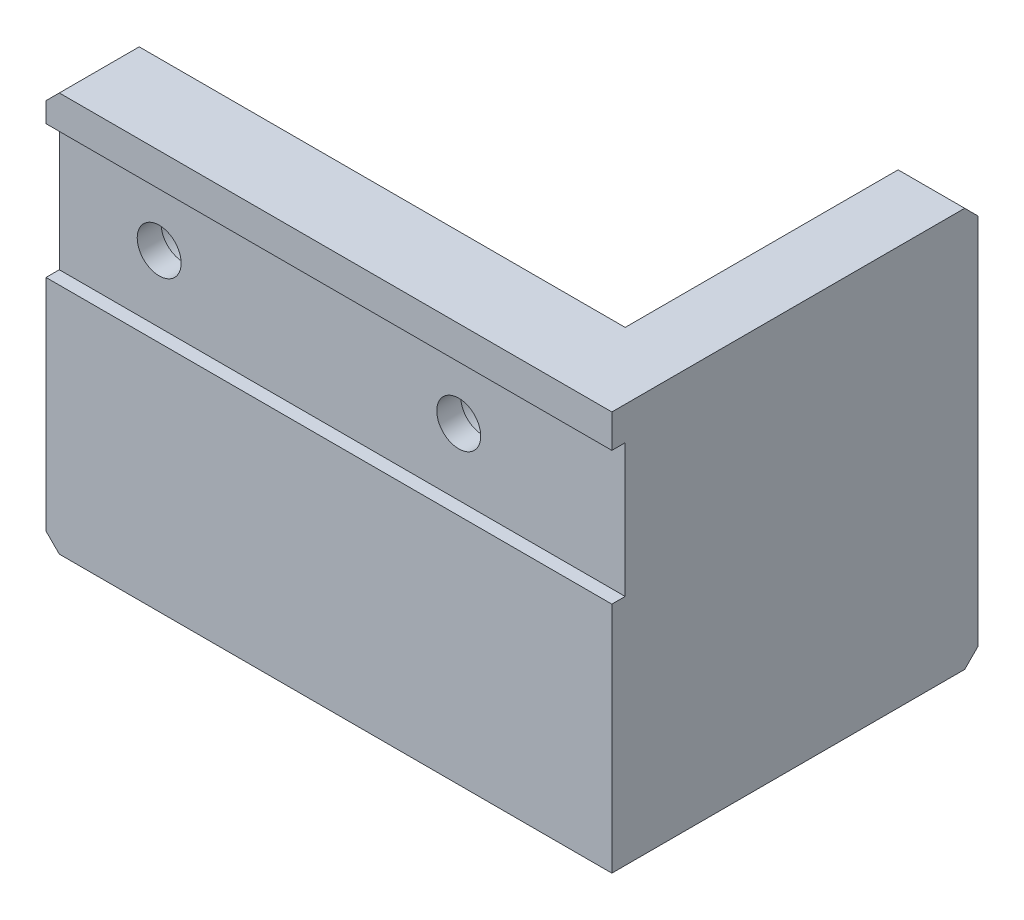
SolidWorks part; units mm, degrees
material "6061-T6"
ref_plane "前视基准面" through (0, 0, 0) normal (0, 0, 1) x (1, 0, 0)
ref_plane "上视基准面" through (0, 0, 0) normal (0, 1, 0) x (1, 0, 0)
ref_plane "右视基准面" through (0, 0, 0) normal (1, 0, 0) x (0, 0, -1)
sketch "草图2" plane through (0, 0, 0) normal (0, 0, 1) x (1, 0, 0)
  line L1 (0, 0) -> (90, 0)
  line L2 (0, 0) -> (0, -60)
  line L3 (0, -60) -> (90, -60)
  line L4 (90, 0) -> (90, -60)
  dimension "D1" = 90
  dimension "D2" = 60
extrude "凸台-拉伸1" add sketch "草图2" along normal blind 12
sketch "草图3" plane through (90, 0, 0) normal (1, 0, 0) x (0, 0, -1)
  line L6 (-12, -60) -> (-12, 0) construction
  line L7 (-12, -5) -> (-10, -5)
  line L8 (-12, -5) -> (-12, -25)
  line L9 (-12, -25) -> (-10, -25)
  line L10 (-10, -5) -> (-10, -25)
  line L12 (-12, 0) -> (0, 0) construction
  dimension "D1" = 2
  dimension "D2" = 5
  dimension "D3" = 20
extrude "切除-拉伸1" cut sketch "草图3" against normal through all
sketch "草图4" plane through (0, 0, 0) normal (0, 1, 0) x (1, 0, 0)
  line L0 (90, 0) -> (0, 0) construction
  line L1 (75, 0) -> (85, 0)
  line L2 (75, 0) -> (75, -1)
  line L3 (75, -1) -> (85, -1)
  line L4 (85, 0) -> (85, -1)
  line L5 (90, -12) -> (90, 0) construction
  dimension "D1" = 1
  dimension "D2" = 5
  dimension "D3" = 10
extrude "切除-拉伸2" cut sketch "草图4" against normal through all
hole_wizard "M6 六角凹头螺钉的柱形沉头孔4" positions "草图5" profile "草图6" counterbore size "M6" standard "ISO"
sketch "草图5" plane through (0, 0, 10) normal (0, 0, 1) x (1, 0, 0)
  line L1 (90, -25) -> (90, -5) construction
  line L2 (80, -15) -> (90, -15) construction
  point P0 (80, -15)
  dimension "D1" = 10
sketch "草图6" plane through (80, -15, 10) normal (1, 0, 0) x (0, -1, 0)
  line L0 (0, 0) -> (0, 18.9828)
  line L1 (0, 18.9828) -> (3.3, 17)
  line L2 (3.3, 17) -> (3.3, 6.4)
  line L3 (3.3, 6.4) -> (5.5, 6.4)
  line L4 (5.5, 6.4) -> (5.5, 0)
  line L5 (5.5, 0) -> (0, 0)
  line L10 (0, 18.9828) -> (-3.3, 17) construction
  line L11 (0, -6.35) -> (0, 107.95) construction
  dimension "孔直径" = 6.6
  dimension "孔深度" = 17
  dimension "柱形沉头孔直径" = 11
  dimension "柱形沉头孔深度" = 6.4
  dimension "导头角度" = 118
hole_wizard "M6 六角凹头螺钉的柱形沉头孔5" positions "草图7" profile "草图8" counterbore size "M6" standard "ISO"
sketch "草图7" plane through (0, 0, 12) normal (0, 0, 1) x (1, 0, 0)
  line L0 (80, -15) -> (80, -45) construction
  line L2 (90, -60) -> (90, -25) construction
  line L3 (0, -60) -> (90, -60) construction
  point P0 (80, -45)
  dimension "D1" = 10
  dimension "D2" = 15
sketch "草图8" plane through (80, -45, 12) normal (1, 0, 0) x (0, -1, 0)
  line L0 (0, 0) -> (0, 18.9828)
  line L1 (0, 18.9828) -> (3.3, 17)
  line L2 (3.3, 17) -> (3.3, 6.4)
  line L3 (3.3, 6.4) -> (5.5, 6.4)
  line L4 (5.5, 6.4) -> (5.5, 0)
  line L5 (5.5, 0) -> (0, 0)
  line L10 (0, 18.9828) -> (-3.3, 17) construction
  line L11 (0, -6.35) -> (0, 107.95) construction
  dimension "孔直径" = 6.6
  dimension "孔深度" = 17
  dimension "柱形沉头孔直径" = 11
  dimension "柱形沉头孔深度" = 6.4
  dimension "导头角度" = 118
hole_wizard "M6 六角凹头螺钉的柱形沉头孔3" positions "草图11" profile "草图12" counterbore size "M6" standard "ISO"
sketch "草图11" plane through (0, 0, 0) normal (0, 0, -1) x (-1, 0, 0)
  line L0 (-60, -15) -> (-15, -15) construction
  line L3 (0, -5) -> (0, -25) construction
  line L6 (0, -5) -> (0, -25) construction
  line L8 (-15, -15) -> (0, -15) construction
  line L10 (-75, -30) -> (0, -30) construction
  line L11 (-75, -60) -> (-75, 0) construction
  line L12 (0, 0) -> (0, -60) construction
  line L14 (-37.5, -30) -> (-37.5, -15) construction
  point P0 (-60, -15)
  point P2 (-15, -15)
  dimension "D1" = 45
sketch "草图12" plane through (60, -15, 0) normal (1, 0, 0) x (0, 1, 0)
  line L0 (0, 0) -> (0, 18.9828)
  line L1 (0, 18.9828) -> (3.3, 17)
  line L2 (3.3, 17) -> (3.3, 6.4)
  line L3 (3.3, 6.4) -> (5.5, 6.4)
  line L4 (5.5, 6.4) -> (5.5, 0)
  line L5 (5.5, 0) -> (0, 0)
  line L10 (0, 18.9828) -> (-3.3, 17) construction
  line L11 (0, -6.35) -> (0, 107.95) construction
  dimension "孔直径" = 6.6
  dimension "孔深度" = 17
  dimension "柱形沉头孔直径" = 11
  dimension "柱形沉头孔深度" = 6.4
  dimension "导头角度" = 118
chamfer "倒角1" distance 2 angle 45 4 edges at (90, 0, 6) (90, -60, 6) (0, -60, 6) (0, 0, 6)
hole_wizard "M3 螺纹孔1" positions "草图13" profile "草图14" tap size "M3" standard "ISO"
sketch "草图13" plane through (0, -60, 0) normal (0, -1, 0) x (-1, 0, 0)
  line L0 (-2, -12) -> (-88, -12) construction
  line L1 (-90, -12) -> (-90, 0) construction
  point P0 (-70, -6)
  dimension "D1" = 6
  dimension "D2" = 20
sketch "草图14" plane through (70, -60, 6) normal (1, 0, 0) x (0, 0, -1)
  line L0 (0, 0) -> (0, 9.2511)
  line L1 (0, 9.2511) -> (1.25, 8.5)
  line L2 (1.25, 8.5) -> (1.25, 0)
  line L5 (1.25, 0) -> (0, 0)
  line L10 (0, 9.2511) -> (-1.25, 8.5) construction
  line L11 (0, -6.35) -> (0, 107.95) construction
  dimension "螺纹孔钻头直径" = 2.5
  dimension "螺纹孔钻头深度" = 8.5
  dimension "导头角度" = 118
cosmetic thread "孔螺蚊线1" parameters "D1"=6, "D2"=3
sketch "草图15" plane through (0, 0, 1) normal (0, 0, -1) x (-1, 0, 0)
  line L1 (-85, 0) -> (-75, 0)
  line L2 (-85, 0) -> (-85, -60)
  line L3 (-85, -60) -> (-75, -60)
  line L4 (-75, 0) -> (-75, -60)
extrude "凸台-拉伸2" add sketch "草图15" along normal blind 44
sketch "草图16" plane through (0, 0, 0) normal (0, 0, -1) x (-1, 0, 0)
  line L0 (-90, -58) -> (-90, -2) construction
  line L1 (-85, -60) -> (-90, -60)
  line L2 (-85, -60) -> (-85, 0)
  line L3 (-85, 0) -> (-90, 0)
  line L4 (-90, -60) -> (-90, 0)
  line L5 (-75, 0) -> (-85, 0) construction
  line L6 (-85, 0) -> (-85, -60) construction
extrude "切除-拉伸3" cut sketch "草图16" against normal through all
hole_wizard "M6 螺纹孔1" positions "草图17" profile "草图18" tap size "M6" standard "ISO"
sketch "草图17" plane through (0, 0, -43) normal (0, 0, -1) x (-1, 0, 0)
  line L0 (-80, -45) -> (-80, -15) construction
  line L2 (-80, -30) -> (-75, -30) construction
  line L3 (-75, -60) -> (-75, 0) construction
  line L5 (-80, -45) -> (-80, -60) construction
  line L6 (-85, -60) -> (-75, -60) construction
  point P0 (-80, -15)
  point P2 (-80, -45)
  dimension "D1" = 15
sketch "草图18" plane through (80, -15, -43) normal (1, 0, 0) x (0, 1, 0)
  line L0 (0, 0) -> (0, 18.5022)
  line L1 (0, 18.5022) -> (2.5, 17)
  line L2 (2.5, 17) -> (2.5, 0)
  line L5 (2.5, 0) -> (0, 0)
  line L10 (0, 18.5022) -> (-2.5, 17) construction
  line L11 (0, -6.35) -> (0, 107.95) construction
  dimension "螺纹孔钻头直径" = 5
  dimension "螺纹孔钻头深度" = 17
  dimension "导头角度" = 118
cosmetic thread "孔螺蚊线2" parameters "D1"=12, "D2"=6
cosmetic thread "孔螺蚊线3" parameters "D1"=12, "D2"=6
chamfer "倒角2" distance 2 angle 45 2 edges at (80, 0, -43) (80, -60, -43)
